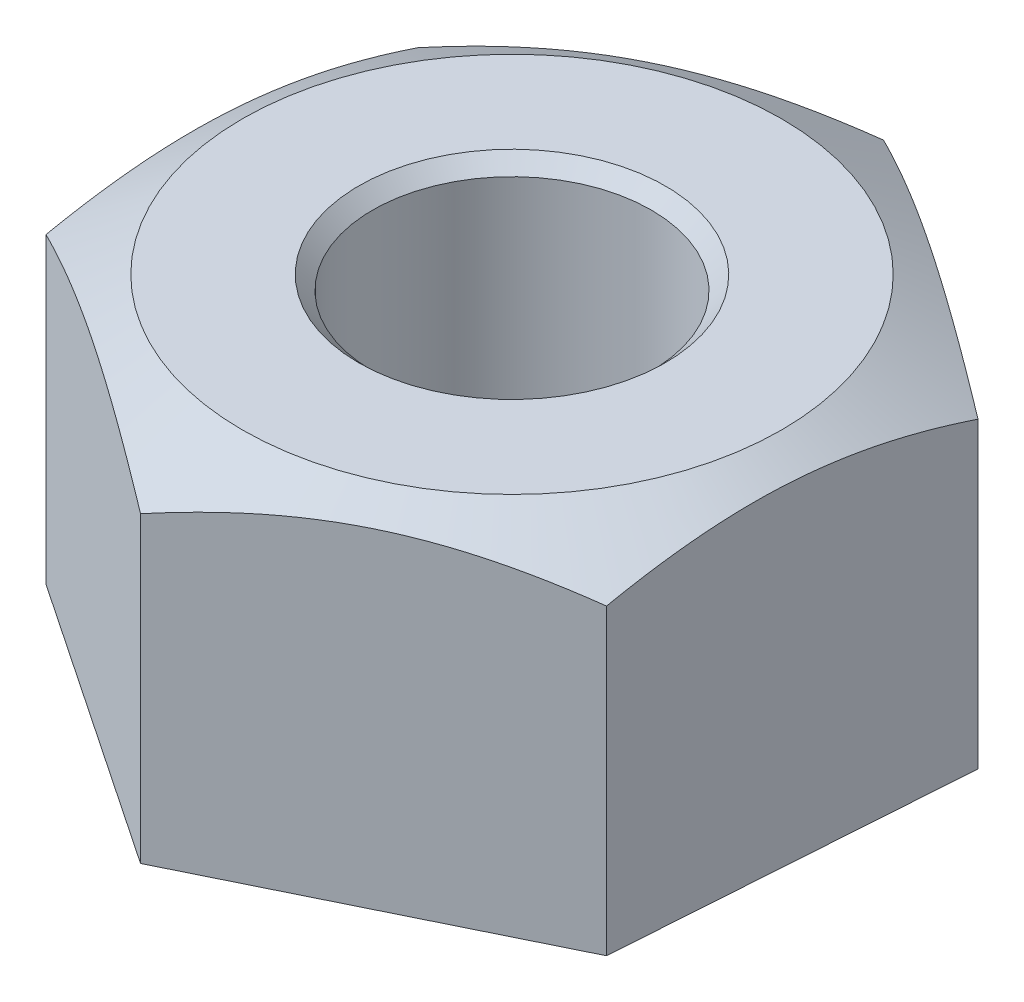
SolidWorks part; units mm, degrees
ref_plane "Front Plane" through (0, 0, 0) normal (0, 0, 1) x (1, 0, 0)
ref_plane "Top Plane" through (0, 0, 0) normal (0, 1, 0) x (1, 0, 0)
ref_plane "Right Plane" through (0, 0, 0) normal (1, 0, 0) x (0, 0, -1)
sketch "Sketch1" plane through (0, 0, 0) normal (0, 1, 0) x (1, 0, 0)
  line L1 (4.1482, -2.7915) -> (4.4916, 2.1967)
  line L2 (4.4916, 2.1967) -> (0.3434, 4.9882)
  line L3 (0.3434, 4.9882) -> (-4.1482, 2.7915)
  line L4 (-4.1482, 2.7915) -> (-4.4916, -2.1967)
  line L5 (-4.4916, -2.1967) -> (-0.3434, -4.9882)
  line L6 (-0.3434, -4.9882) -> (4.1482, -2.7915)
  circle A0 centre (0, 0) radius 4.3301 construction
  circle A1 centre (0, 0) radius 2
  dimension "D1" = 4
  dimension "D2" = 10
extrude "Boss-Extrude1" add sketch "Sketch1" along normal blind 5
sketch "Sketch8" plane through (0, 5, 0) normal (0, 1, 0) x (1, 0, 0)
  circle A0 centre (0, 0) radius 3.8691
extrude "Cut-Extrude1" cut sketch "Sketch8" against normal blind 5 draft 60 flip side to cut
chamfer "Chamfer1" distance 0.2 angle 45 1 edges at (0, 5, 2)
chamfer "Chamfer2" distance 0.2 angle 45 1 edges at (0, 0, 2)
